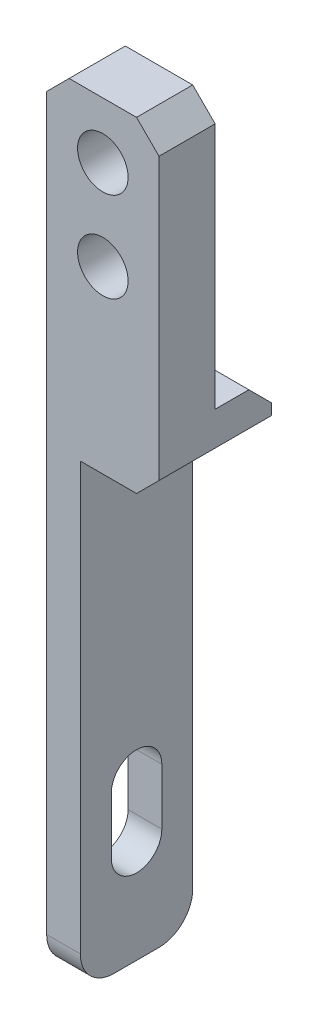
from build123d import *

# Parameters (mm, degrees)
SKETCH1_W            = 10
SKETCH1_H            = 70
BOSS_EXTRUDE1_DEPTH  = 5
SKETCH2_W            = 7
SKETCH2_H            = 41
CUT_EXTRUDE1_DEPTH   = 37.742346142
SKETCH3_W            = 5
SKETCH3_H            = 24
CUT_EXTRUDE2_DEPTH   = 37.742346142
CUT_EXTRUDE3_DEPTH   = 37.742346142
FILLET1_R            = 3
M4_CLEARANCE_HOLE1_D = 4.5
CHAMFER1_SIZE        = 2


with BuildPart() as part:
    # Sketch1 → Boss-Extrude1 (new, symmetric)
    with BuildSketch(Plane.XY):
        Rectangle(SKETCH1_W, SKETCH1_H)
    extrude(amount=BOSS_EXTRUDE1_DEPTH, both=True)

    # Sketch2 → Cut-Extrude1 (cut, through all)
    with BuildSketch(Plane.XY.offset(5)):
        with Locations((1.5, -14.5)):
            Rectangle(SKETCH2_W, SKETCH2_H)
    extrude(amount=-CUT_EXTRUDE1_DEPTH, mode=Mode.SUBTRACT)

    # Sketch3 → Cut-Extrude2 (cut, through all)
    with BuildSketch(Plane(origin=(5, 0, 0), x_dir=(0, 0, -1), z_dir=(1, 0, 0))):
        with Locations((2.5, 23)):
            Rectangle(SKETCH3_W, SKETCH3_H)
    extrude(amount=-CUT_EXTRUDE2_DEPTH, mode=Mode.SUBTRACT)

    # Sketch4 → Cut-Extrude3 (cut, through all)
    with BuildSketch(Plane.ZY.offset(5)):
        with BuildLine():
            Line((2.25, -21), (2.25, -26))
            ThreePointArc((2.25, -26), (0, -28.25), (-2.25, -26))
            Line((-2.25, -26), (-2.25, -21))
            ThreePointArc((-2.25, -21), (0, -18.75), (2.25, -21))
        make_face()
    extrude(amount=-CUT_EXTRUDE3_DEPTH, mode=Mode.SUBTRACT)

    # Fillet1
    fillet1_edges = [part.edges().sort_by_distance(p)[0] for p in [
        (-3.5, -35, 5),
        (-3.5, -35, -5),
    ]]
    fillet(fillet1_edges, radius=FILLET1_R)

    # M4 Clearance Hole1 (through all)
    with Locations(Plane.XY.offset(5)):
        with Locations((0, 30), (0, 22)):
            Hole(M4_CLEARANCE_HOLE1_D / 2)

    # Chamfer1
    chamfer1_edges = [part.edges().sort_by_distance(p)[0] for p in [
        (5, 6, 0),
        (0, 11, -5),
        (-5, 35, 2.5),
        (5, 35, 2.5),
    ]]
    chamfer(chamfer1_edges, length=CHAMFER1_SIZE)


solid = part.part
